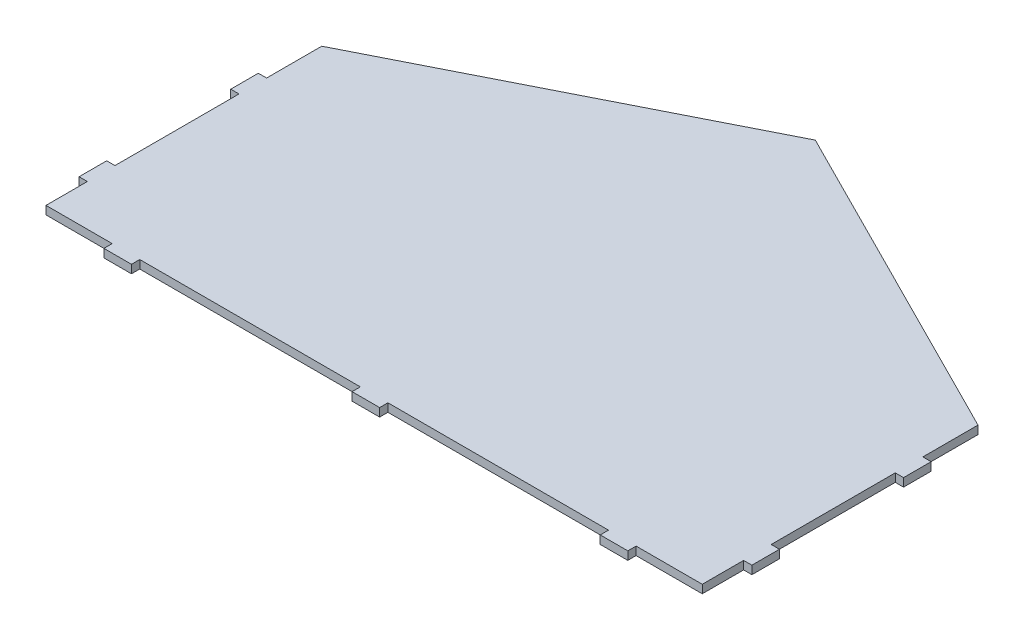
SolidWorks part; units mm, degrees
ref_plane "Front Plane" through (0, 0, 0) normal (0, 0, 1) x (1, 0, 0)
ref_plane "Top Plane" through (0, 0, 0) normal (0, 1, 0) x (1, 0, 0)
ref_plane "Right Plane" through (0, 0, 0) normal (1, 0, 0) x (0, 0, -1)
sketch "Sketch1" plane through (0, 0, 0) normal (0, 1, 0) x (1, 0, 0)
  line L0 (-119, 50) -> (0, 110)
  line L1 (-119, -50) -> (119, -50)
  line L2 (-119, -50) -> (-119, 50)
  line L4 (119, -50) -> (119, 50)
  line L5 (-119, -50) -> (119, 50) construction
  line L6 (-119, 50) -> (119, -50) construction
  line L7 (0, 110) -> (119, 50)
  point P0 (0, 0)
  dimension "D1" = 238
  dimension "D2" = 100
  dimension "D3" = 60
  dimension "D4" = 119
extrude "Boss-Extrude1" add sketch "Sketch1" along normal blind 3
sketch "Sketch3" plane through (0, 3, 0) normal (0, 1, 0) x (1, 0, 0)
  line L0 (119, -50) -> (119, 50) construction
  line L1 (119, 30) -> (122, 30)
  line L2 (119, 30) -> (119, 20)
  line L3 (119, 20) -> (122, 20)
  line L4 (122, 30) -> (122, 20)
  line L5 (0, -1000) -> (0, 49000) construction
  line L6 (119, -35) -> (122, -35)
  line L7 (119, -35) -> (119, -25)
  line L8 (119, -25) -> (122, -25)
  line L9 (122, -35) -> (122, -25)
  line L10 (-119, -50) -> (119, -50) construction
  line L11 (-122, -35) -> (-122, -25)
  line L12 (-119, -25) -> (-122, -25)
  line L13 (-119, -35) -> (-119, -25)
  line L14 (-119, -35) -> (-122, -35)
  line L15 (-122, 30) -> (-122, 20)
  line L16 (-119, 20) -> (-122, 20)
  line L17 (-119, 30) -> (-119, 20)
  line L18 (-119, 30) -> (-122, 30)
  line L19 (-95, -50) -> (-95, -53)
  line L20 (85, -50) -> (95, -50)
  line L21 (85, -50) -> (85, -53)
  line L22 (85, -53) -> (95, -53)
  line L23 (95, -50) -> (95, -53)
  line L24 (-85, -53) -> (-95, -53)
  line L25 (-85, -50) -> (-85, -53)
  line L26 (-85, -50) -> (-95, -50)
  line L28 (-5, -53) -> (5, -53)
  line L29 (-5, -53) -> (-5, -50)
  line L30 (-5, -50) -> (5, -50)
  line L31 (5, -53) -> (5, -50)
  line L32 (-5, -53) -> (5, -50) construction
  line L33 (-5, -50) -> (5, -53) construction
  point P31 (0, -51.5)
  dimension "D1" = 3
  dimension "D2" = 10
  dimension "D3" = 70
  dimension "D4" = 10
  dimension "D5" = 3
  dimension "D6" = 15
  dimension "D7" = 10
  dimension "D8" = 3
  dimension "D9" = 24
  dimension "D10" = 3
  dimension "D11" = 10
extrude "Boss-Extrude2" add sketch "Sketch3" against normal up to surface (3 mm away) up to face at (0, 0, -22)
